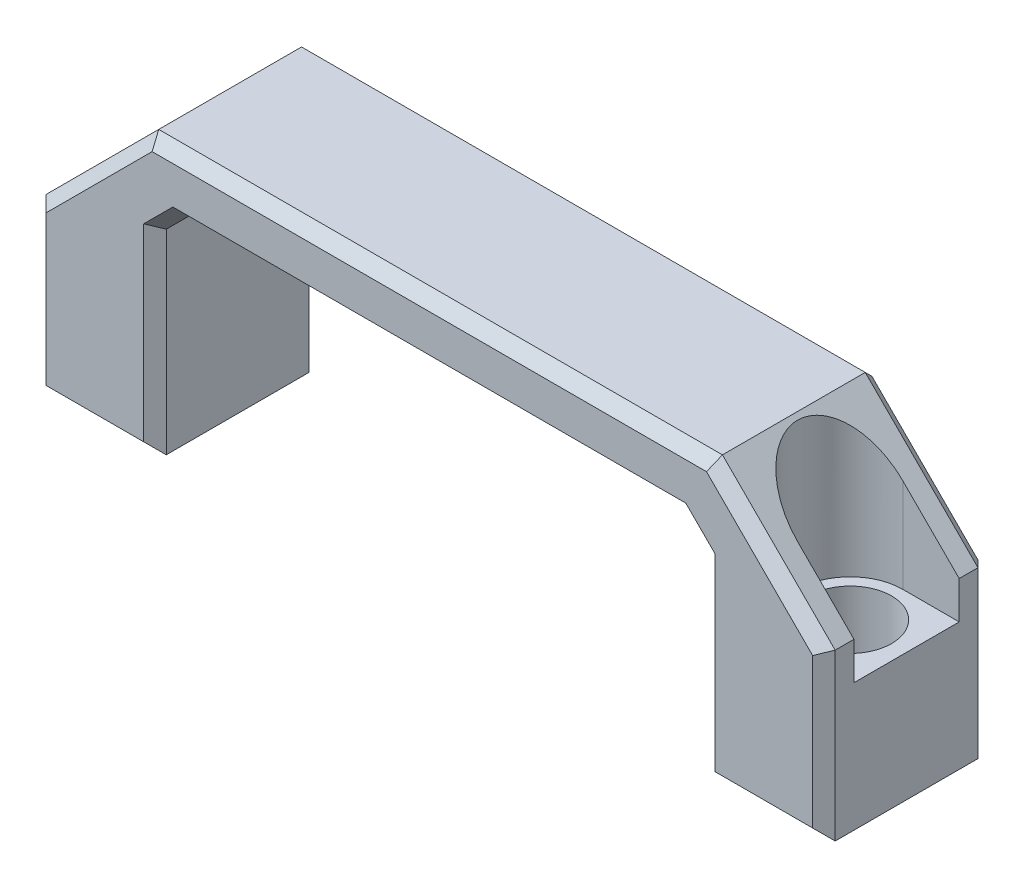
SolidWorks part; units mm, degrees
ref_plane "前视" through (0, 0, 0) normal (0, 0, 1) x (1, 0, 0)
ref_plane "上视" through (0, 0, 0) normal (0, 1, 0) x (1, 0, 0)
ref_plane "右视" through (0, 0, 0) normal (1, 0, 0) x (0, 0, -1)
sketch "草图1" plane through (0, 0, 0) normal (0, 0, 1) x (1, 0, 0)
  line L0 (-52.5, 0) -> (-36.5, 0)
  line L1 (-36.5, 0) -> (-36.5, 26)
  line L2 (-33.5, 29) -> (33.5, 29)
  line L3 (36.5, 26) -> (36.5, 0)
  line L4 (36.5, 0) -> (52.5, 0)
  line L5 (52.5, 0) -> (52.5, 22)
  line L6 (37.5, 37) -> (-37.5, 37)
  line L7 (-52.5, 22) -> (-52.5, 0)
  line L8 (0, 0) -> (0, 63.1256) construction
  line L9 (33.5, 29) -> (36.5, 26)
  line L10 (-36.5, 26) -> (-33.5, 29)
  line L11 (-37.5, 37) -> (-52.5, 22)
  line L12 (52.5, 22) -> (37.5, 37)
  point P3 (-36.5, 29)
  point P4 (36.5, 29)
  point P7 (52.5, 37)
  point P8 (-52.5, 37)
  dimension "D1" = 37
  dimension "D2" = 105
  dimension "D3" = 8
  dimension "D4" = 16
extrude "凸台-拉伸1" add sketch "草图1" along normal mid plane 22
hole_wizard "M6 六角凹头螺钉的柱形沉头孔1" positions "草图3" profile "草图2" counterbore size "M6" standard "Iso" end condition through all
sketch "草图3" plane through (0, 37, 0) normal (0, 1, 0) x (1, 0, 0)
  line L0 (0, 0) -> (0, -24.3527) construction
  point P0 (-45, 0)
  point P7 (45, 0)
  dimension "D1" = 90
sketch "草图2" plane through (-45, 37, 0) normal (1, 0, 0) x (0, 0, 1)
  line L0 (0, 0) -> (0, 37)
  line L1 (0, 37) -> (3.25, 37)
  line L3 (3.25, 37) -> (3.25, 30)
  line L4 (3.25, 30) -> (5.5, 30)
  line L5 (5.5, 30) -> (5.5, 0)
  line L7 (5.5, 0) -> (0, 0)
  line L11 (0, -6.35) -> (0, 107.95) construction
  dimension "通孔孔直径" = 6.5
  dimension "通孔孔深度" = 37
  dimension "柱形沉头孔直径" = 11
  dimension "柱形沉头孔深度" = 30
sketch "草图4" plane through (0, 37, 0) normal (0, 1, 0) x (1, 0, 0)
  line L0 (-52.5, 0) -> (-45, 0) construction
  line L1 (-52.5, -11) -> (-52.5, 11) construction
  line L2 (-52.5, 7) -> (-45, 7)
  line L3 (-52.5, -7) -> (-45, -7)
  line L4 (0, 0) -> (0, 20.2277) construction
  line L5 (52.5, 0) -> (45, 0) construction
  line L6 (52.5, 7) -> (45, 7)
  line L7 (52.5, -7) -> (45, -7)
  arc A0 (-52.5, 7) -> (-52.5, -7) centre (-52.5, 0) ccw
  arc A1 (-45, -7) -> (-45, 7) centre (-45, 0) ccw
  arc A2 (52.5, 7) -> (52.5, -7) centre (52.5, 0) cw
  arc A3 (45, -7) -> (45, 7) centre (45, 0) cw
  point P5 (-48.75, 0)
  point P15 (48.75, 0)
  dimension "D1" = 14
extrude "切除-拉伸1" cut sketch "草图4" against normal blind 20
chamfer "倒角1" distance 1.5 angle 45 24 edges at (-44.5, 0, -11) (-36.5, 13, -11) (-35, 27.5, -11) (0, 29, -11) (35, 27.5, -11) (36.5, 13, -11) (44.5, 0, -11) (52.5, 11, -11) (45, 29.5, -11) (0, 37, -11) (-45, 29.5, -11) (-52.5, 11, -11) (-45, 29.5, 11) (0, 37, 11) (45, 29.5, 11) (52.5, 11, 11) (44.5, 0, 11) (36.5, 13, 11) (35, 27.5, 11) (0, 29, 11) (-35, 27.5, 11) (-36.5, 13, 11) (-44.5, 0, 11) (-52.5, 11, 11)
